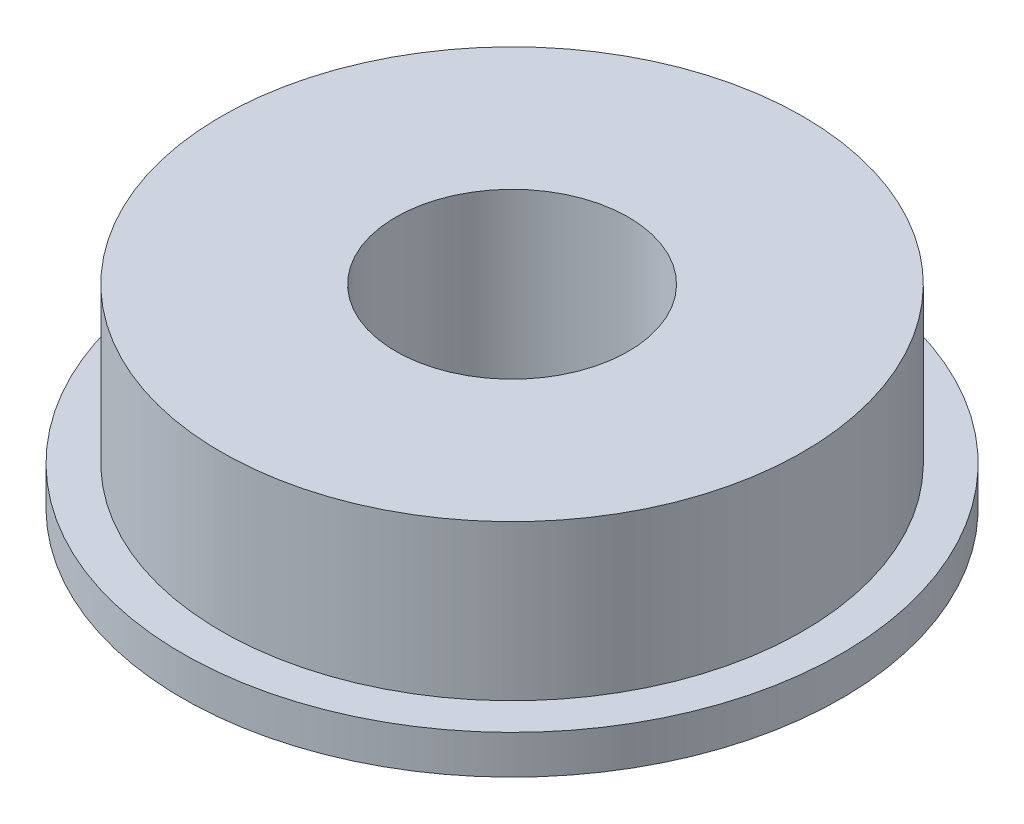
from build123d import *


with BuildPart() as part:
    # 草图1 → 旋转1 (revolve)
    with BuildSketch(Plane.XY, mode=Mode.PRIVATE) as revolve_1_sk:
        Polygon((3, 2.31741573), (7.5, 2.31741573), (7.5, -1.68258427), (8.5, -1.68258427), (8.5, -2.68258427), (3, -2.68258427), align=None)
    revolve(revolve_1_sk.sketch.rotate(Axis((0, 0, 0), (0, 1, 0)), 90), axis=Axis((0, 0, 0), (0, 1, 0)))


solid = part.part
